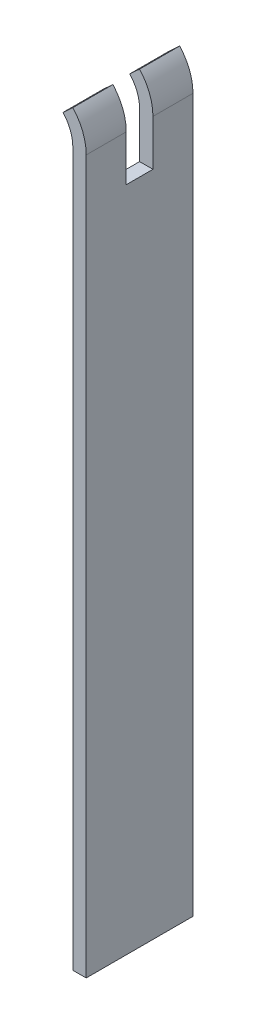
SolidWorks part; units mm, degrees
ref_plane "前视基准面" through (0, 0, 0) normal (0, 0, 1) x (1, 0, 0)
ref_plane "上视基准面" through (0, 0, 0) normal (0, 1, 0) x (1, 0, 0)
ref_plane "右视基准面" through (0, 0, 0) normal (1, 0, 0) x (0, 0, -1)
sketch "草图1" plane through (0, 0, 0) normal (0, 0, 1) x (1, 0, 0)
  line L0 (0, 0) -> (5, 0)
  line L1 (5, 0) -> (5, 261)
  line L2 (-3.6842, 270.4649) -> (0, 273.8452)
  line L3 (0, 0) -> (0, 261)
  arc A0 (5, 261) -> (0, 273.8452) centre (-14, 261) ccw
  arc A1 (0, 261) -> (-3.6842, 270.4649) centre (-14, 261) ccw
  dimension "D1" = 19
  dimension "D2" = 5
extrude "凸台-拉伸1" add sketch "草图1" along normal blind 40
sketch "草图2" plane through (5, 0, 0) normal (1, 0, 0) x (0, 0, -1)
  line L0 (-20, 273.8452) -> (-25, 273.8452)
  line L1 (-40, 273.8452) -> (0, 273.8452) construction
  line L2 (-20, 273.8452) -> (-15, 273.8452)
  line L3 (-15, 273.8452) -> (-15, 243.8452)
  line L4 (-15, 243.8452) -> (-25, 243.8452)
  line L5 (-25, 243.8452) -> (-25, 273.8452)
extrude "切除-拉伸1" cut sketch "草图2" against normal blind 40
sketch "草图3" plane through (0, 0, 0) normal (0, -1, 0) x (1, 0, 0)
  line L8 (0, 0) -> (5, 0)
  line L9 (5, 0) -> (5, 40)
  line L10 (5, 40) -> (0, 40)
  line L11 (0, 40) -> (0, 0)
  line L12 (0, 0) -> (5, 0)
  line L13 (5, 0) -> (5, 40)
  line L14 (5, 40) -> (0, 40)
  line L15 (0, 40) -> (0, 0)
  dimension "D1" = 0
extrude "凸台-拉伸3" add sketch "草图3" along normal blind 6
